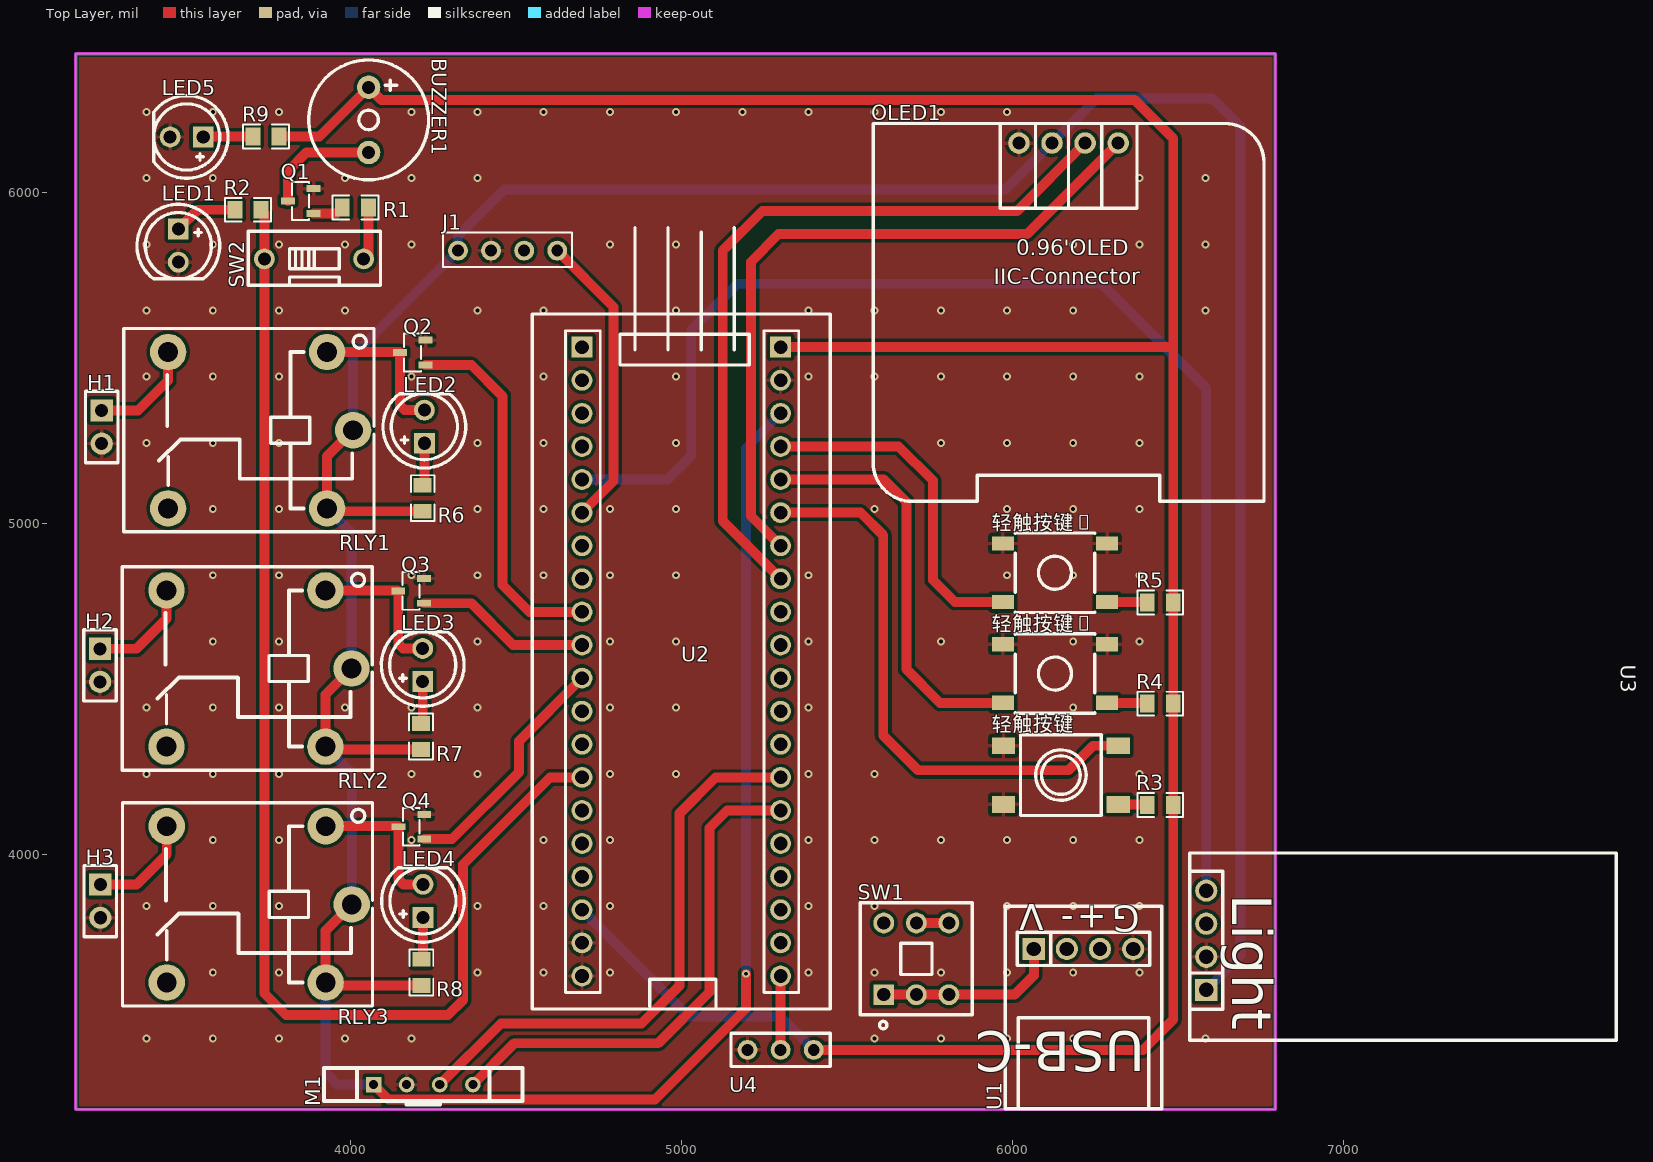
[diagram p0: Top Layer view]
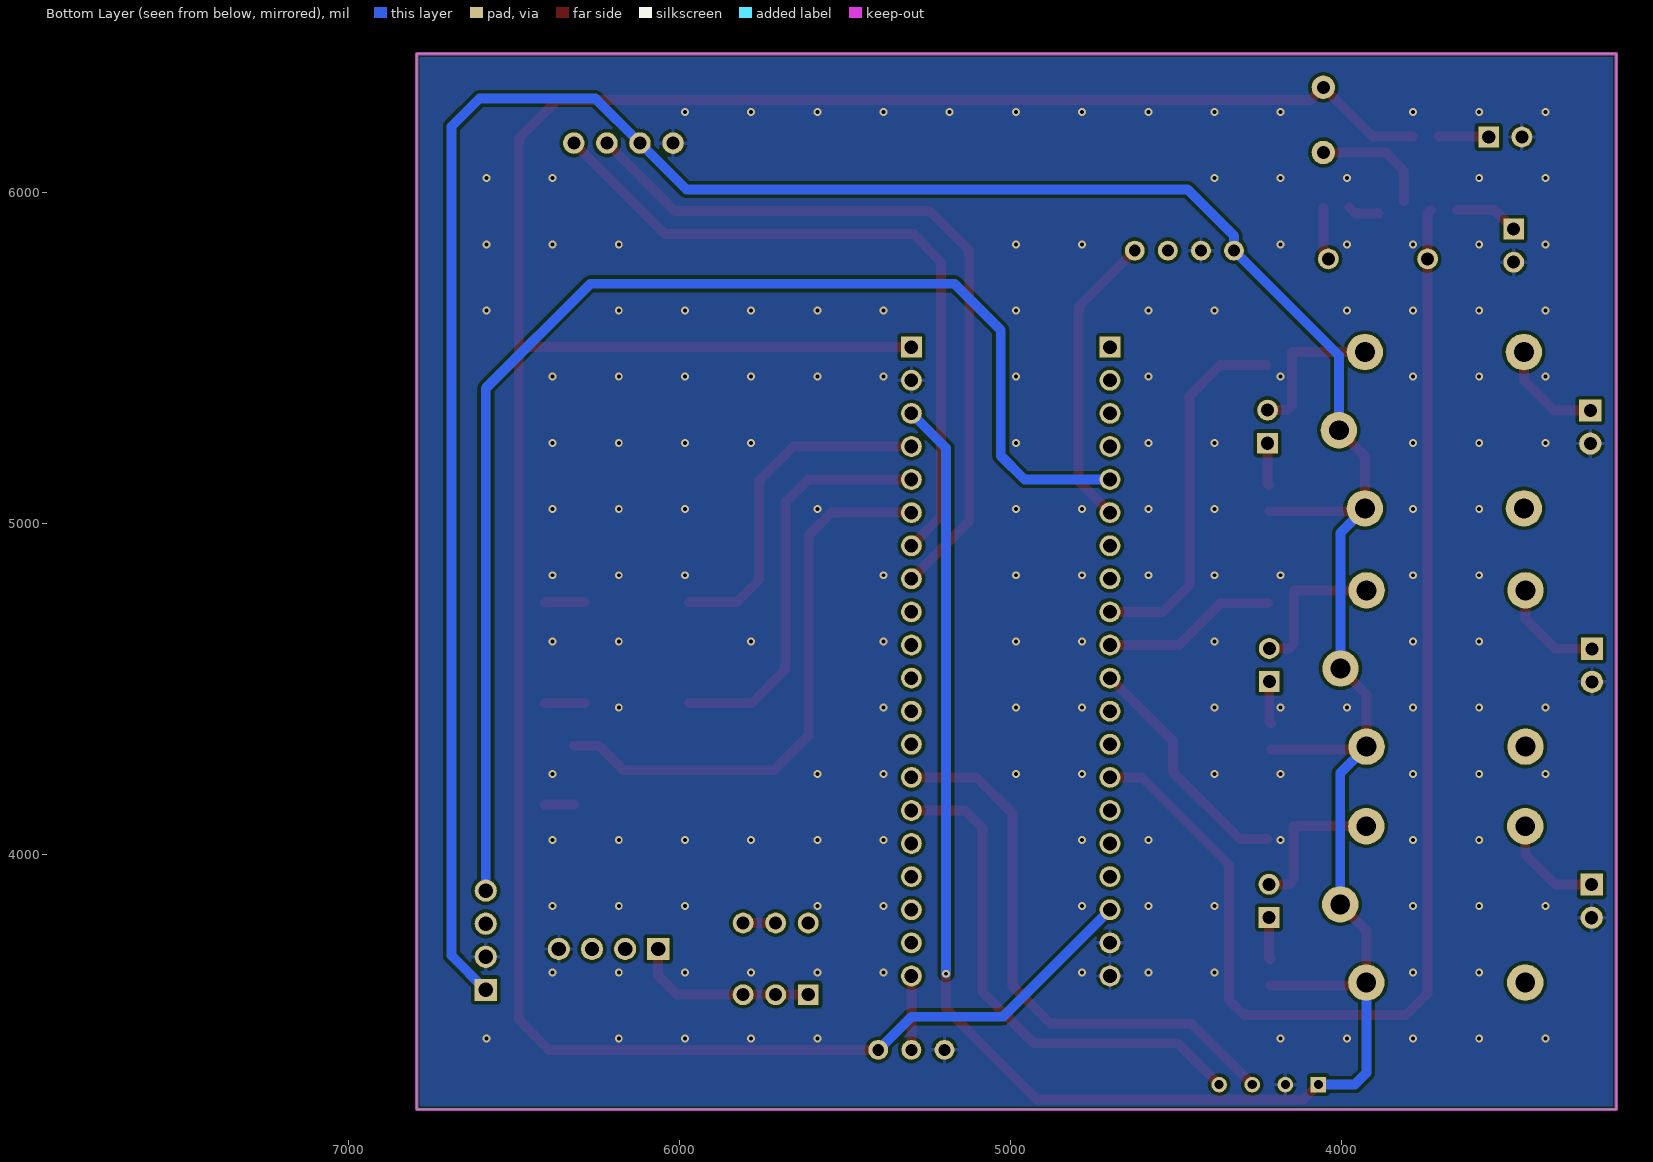
[diagram p1: Bottom Layer view, seen from below]
# Altium PCB MISC51322.pcbdoc
Units mil, origin at the board's own origin, x right, y up, seen from the top; angles counter-clockwise.
Board outline 3625 x 3190 mil, 2 copper layers (Top Layer, Bottom Layer), stack 62.206 mil thick; 37 components, 36 nets, 146 pads, 159 vias.

## Layer stack, top to bottom
Top Solder Mask Layer: solder mask 0.394, Dk 3.3
Top Layer: signal copper 1.379
Dielectric1: surface 59.449, FR4, Dk 4.5
Bottom Layer: signal copper 1.378
Bottom Solder Mask Layer: solder mask 0.394, Dk 3.3

## Board outline
3170,6420 3170,3230 6795,3230 6795,6420

## Design rules (kind name [scope] priority, off if disabled: settings)
BoardOutlineClearance copperThickness2oz_1 [All] p2 off: genericclearance=7.99 ignorepadtopadclearanceinfootprint=FALSE except(0: Arc-SplitContinuation Track-SplitContinuation SMDPad-SplitContinuation THPad-SplitContinuation Via-SplitContinuation Fill-SplitContinuation Region-SplitContinuation Poly-SplitContinuation Text-SplitContinuation Hole-SplitContinuation; 5.98: Arc-CutoutEdge SMDPad-CutoutEdge THPad-CutoutEdge Via-CutoutEdge Fill-CutoutEdge Region-CutoutEdge Text-CutoutEdge; 6.93: Hole-OutlineEdge Hole-CutoutEdge; 10: Poly-OutlineEdge Poly-CutoutEdge; 11.81: Arc-OutlineEdge Track-OutlineEdge SMDPad-OutlineEdge THPad-OutlineEdge Via-OutlineEdge Fill-OutlineEdge Region-OutlineEdge Text-OutlineEdge Track-CutoutEdge)
BoardOutlineClearance copperThickness1oz_1 [All] p4: genericclearance=4.02 ignorepadtopadclearanceinfootprint=FALSE except(0: Arc-SplitContinuation Track-SplitContinuation SMDPad-SplitContinuation THPad-SplitContinuation Via-SplitContinuation Fill-SplitContinuation Region-SplitContinuation Poly-SplitContinuation Text-SplitContinuation Hole-SplitContinuation; 6: SMDPad-CutoutEdge THPad-CutoutEdge Via-CutoutEdge Fill-CutoutEdge Region-CutoutEdge Text-CutoutEdge; 6.93: Hole-OutlineEdge Hole-CutoutEdge; 10: Poly-OutlineEdge Poly-CutoutEdge; 11.8: Arc-OutlineEdge Track-OutlineEdge SMDPad-OutlineEdge THPad-OutlineEdge Via-OutlineEdge Fill-OutlineEdge Region-OutlineEdge Text-OutlineEdge; 11.81: Arc-CutoutEdge Track-CutoutEdge)
Clearance copperThickness2oz [All] p1 off: gap=7.99 ignorepadtopadclearanceinfootprint=FALSE except(5.98: SMDPad-Track SMDPad-SMDPad THPad-Track SMDPad-THPad THPad-THPad Track-Via SMDPad-Via THPad-Via Via-Via Fill-Track Region-Track Fill-SMDPad Region-SMDPad Fill-THPad Region-THPad Fill-Via Region-Via Fill-Fill Fill-Region Region-Region Arc-Track Arc-SMDPad Arc-THPad Arc-Via Fill-Arc Region-Arc Arc-Arc Text-Track SMDPad-Text Text-THPad Text-Via Fill-Text Region-Text Arc-Text Text-Text; 6.93: Hole-Track Hole-SMDPad Hole-THPad Hole-Via Fill-Hole Region-Hole Hole-Arc Hole-Text; 10: Poly-Track Poly-SMDPad Poly-THPad Poly-Via Poly-Fill Poly-Region Poly-Poly Poly-Arc Poly-Text Poly-Hole)
Clearance copperThickness1oz [All] p3: gap=4.02 ignorepadtopadclearanceinfootprint=FALSE except(5.98: SMDPad-Track SMDPad-SMDPad THPad-Track SMDPad-THPad THPad-THPad Track-Via SMDPad-Via THPad-Via Via-Via Fill-Track Region-Track Fill-SMDPad Region-SMDPad Fill-THPad Region-THPad Fill-Via Region-Via Fill-Fill Fill-Region Region-Region; 6: Arc-Track Arc-SMDPad Arc-THPad Arc-Via Fill-Arc Region-Arc Arc-Arc Text-Track SMDPad-Text Text-THPad Text-Via Fill-Text Region-Text Arc-Text Text-Text; 6.93: Hole-Track Hole-SMDPad Hole-THPad Hole-Via Fill-Hole Region-Hole Hole-Arc Hole-Text; 10: Poly-Track Poly-SMDPad Poly-THPad Poly-Via Poly-Fill Poly-Region Poly-Poly Poly-Arc Poly-Text Poly-Hole)
DiffPairsRouting differentialPair [All] p1: maxlimit=6 minlimit=6 mostfreqgap=6 toplayer_minwidth=5 toplayer_prefwidth=10 toplayer_maxwidth=100 toplayer_mingap=6 toplayer_prefgap=6 toplayer_maxgap=6 bottomlayer_minwidth=5 bottomlayer_prefwidth=10 bottomlayer_maxwidth=100 bottomlayer_mingap=6 bottomlayer_prefgap=6 bottomlayer_maxgap=6 maxuncoupledlength=10
HoleToHoleClearance otherClearance [All] p1: gap=11.81 allowstackedmicrovias=TRUE
Length netLength [All] p1: minlimit=0 maxlimit=0
MatchedLengths netLengthTolerance [All] p1: tolerance=1000
PasteMaskExpansion pasteMaskExpansion [All] p1: expansion=0
PlaneConnect innerPlane [All] p1: planeconnectstyle=Relief reliefexpansion=20 reliefentries=4 reliefconductorwidth=10 reliefairgap=10
PolygonConnect copperRegion [(InNet('GND'))] p1: connectstyle=Relief reliefconductorwidth=10 reliefentries=4 polygonreliefangle="90 Angle" airgapwidth=10 via.connectstyle=Relief via.reliefconductorwidth=10 via.reliefentries=4 via.polygonreliefangle="90 Angle" via.airgapwidth=10
RoutingVias viaSize [All] p1: holewidth=12.01 width=24.02 viastyle="Through Hole" minholewidth=11.81 minwidth=19.68 maxholewidth=248.03 maxwidth=393.7
SolderMaskExpansion solderMaskExpansion [IsVia] p1: expansion=-1000 istentingtop=TRUE
SolderMaskExpansion solderMaskExpansion [All] p2: expansion=2 istentingtop=FALSE
Width copperThickness2oz_2 [All] p1 off: maxlimit=100 minlimit=8 preferedwidth=10
Width copperThickness1oz_2 [All] p2: maxlimit=100 minlimit=5 preferedwidth=10

## Components (designator, comment, footprint, x,y, rotation, side; value= is the part's Value field where it differs from the comment)
BUZZER1 "3kHz" BUZ-TH_BD9.0-P5.00-D0.6-FD 4055,6220 r270 top
H1 "" HDR-TH_2P-P2.54-V-F 3248.48,5291.97 r270 top
H2 "" HDR-TH_2P-P2.54-V-F 3243.48,4571.97 r270 top
H3 "" HDR-TH_2P-P2.54-V-F 3244.21,3859.22 r270 top
J1 "土壤湿度传感器模块" Hearder-4 4325,5825 r0 top
LED1 "" LED-TH_5mm 3480,5840 r270 top
LED2 "" LED-TH_5mm 4223.48,5293.03 r90 top
LED3 "" LED-TH_5mm 4218.48,4573.03 r90 top
LED4 "" LED-TH_5mm 4219.21,3860.28 r90 top
LED5 "" LED-TH_5mm 3505.35,6168.51 r180 top
M1 "BT06" BT06 4070,3305 r90 top
OLED1 "" 0.96OLED_4P 6170,6150 r0 top
Q1 "S8050" SOT-23-3_L2.9-W1.3-P1.90-LS2.3-BR 3850,5975 r0 top
Q2 "S8050" SOT-23-3_L2.9-W1.3-P1.90-LS2.3-BR 4188.48,5516.97 r0 top
Q3 "S8050" SOT-23-3_L2.9-W1.3-P1.90-LS2.3-BR 4183.48,4796.97 r0 top
Q4 "S8050" SOT-23-3_L2.9-W1.3-P1.90-LS2.3-BR 4184.21,4084.22 r0 top
R1 "1K" R0805 4015,5955 r180 top
R2 "1K" R0805 3690.35,5948.51 r0 top
R3 "10K" R0805 6446.93,4150.32 r0 top
R4 "10K" R0805 6446.93,4456.02 r0 top
R5 "10K" R0805 6446.93,4761.73 r0 top
R6 "1K" R0805 4218.48,5076.97 r90 top
R7 "1K" R0805 4213.48,4356.97 r90 top
R8 "1K" R0805 4214.21,3644.22 r90 top
R9 "1K" R0805 3745,6170 r0 top
RLY1 "SRD-05VDC-SL-C" RELAY-TH_SRD-XXVDC-XL-C 3728.75,5282.36 r180 top
RLY2 "SRD-05VDC-SL-C" RELAY-TH_SRD-XXVDC-XL-C 3723.75,4562.36 r180 top
RLY3 "SRD-05VDC-SL-C" RELAY-TH_SRD-XXVDC-XL-C 3724.48,3849.61 r180 top
SW1 "自锁开关" SW-TH_6P-L8.5-W8.5-P2.50-LS5.5-BL-2 5710,3685 r0 top
SW2 "拨码" SW-TH_DSWB01LHGET 3890,5800 r90 top
U1 "" USB-type-C模块 6215,3715 r90 top
U2 "CW32F030C8最小系统板" STM32F103C8T6核心板 4999.86,4583.38 r0 top
U3 "" 光敏传感器模块 6535,3735 r270 top
U4 "DS18B20" 3p_2.54 5300,3410 r0 top
轻触按键 "SH-6X6X6.5H-TP" SW-SMD_4P-L6.2-W6.2-P4.50-LS9.5-TL 6146.68,4240.32 r0 top
轻触按键1 "SH-6X6X6.5H-TP" SW-SMD_4P-L6.0-W6.0-P4.50-LS8.8 6128.96,4547.05 r0 top
轻触按键2 "SH-6X6X6.5H-TP" SW-SMD_4P-L6.0-W6.0-P4.50-LS8.8 6128.96,4851.73 r0 top

## Footprints (in the part's own frame and the unit in brackets; to place one, negate y for a bottom-side part, rotate by r counter-clockwise, add the part's x,y. Pads: shape width x height; smd on the part's side, far side on the other; paste and mask are expansions set on the pad)
0.96OLED_4P [mm]
  round 1.65 hole 1 copper offset 0,0: 1(-3.81,-0.001) 2(-1.27,0.002) 3(1.27,0.002) 4(3.81,0.002)
  silkscreen extent -15,-27.5 15,1.5
3p_2.54 [mil]
  round 60 hole 36: 1(-100,0) 2(0,0) 3(100,0)
  silkscreen extent -150,-50 150,50
BT06 [mm]
  rect 1.2x1.2 hole 0.7: 1(0,0)
  round 1.2 hole 0.7: 2(0,-2.54) 3(0,-5.08) 4(0,-7.62)
  silkscreen extent -1.52,-11.43 1.27,3.81
BUZ-TH_BD9.0-P5.00-D0.6-FD [mm]
  round 1.8 hole 1 copper offset 0,0: 1(-2.5,0)
  round 1.8 hole 1: 2(2.5,0)
  silkscreen extent -4.6,-4.6 4.6,4.6
HDR-TH_2P-P2.54-V-F [mm]
  rect 1.7x1.7 hole 1: 1(-1.27,0)
  round 1.7 hole 1: 2(1.27,0)
  silkscreen extent -2.74,-1.25 2.74,1.25
Hearder-4 [mil]
  round 60 hole 36: 1(0,0) 2(100,0) 3(200,0) 4(300,0)
  silkscreen extent -45,-50 345,55
LED-TH_5mm [mm]
  rect 1.6x1.6 hole 1 paste+0 mask+0.051: 1(-1.27,0)
  round 1.6 hole 1 paste+0 mask+0.051: 2(1.27,0)
  silkscreen extent -3.17,-3.17 2.54,3.17
R0805 [mm]
  rect 1.133x1.377 smd paste-100 mask+0.051: 1(-1,0) 2(1,0)
  silkscreen extent -1.76,-0.92 1.76,0.92
RELAY-TH_SRD-XXVDC-XL-C [mil]
  round 110 hole 60: 1(-200.79,-236.22) 2(279.53,-236.2) 3(279.53,236.2) 4(-200.79,236.22) 5(-279.53,0)
  silkscreen extent -342,-307 413,307
SOT-23-3_L2.9-W1.3-P1.90-LS2.3-BR [mm]
  rect 1.07x0.532 smd: 1(0.99,-0.95) 2(0.99,0.95) 3(-0.99,0)
  silkscreen extent -0.66,-1.45 0.64,1.45
STM32F103C8T6核心板 [mil]
  rect 63x63 hole 41.3 paste+4 mask+4: 1(-300,950) 40(300,950)
  round 63 hole 41.3 paste+4 mask+4: 2(-300,850) 3(-300,750) 4(-300,650) 5(-300,550) 6(-300,450) 7(-300,350) 8(-300,250) 9(-300,150) 10(-300,50) 11(-300,-50) 12(-300,-150) 13(-300,-250) 14(-300,-350) 15(-300,-450) 16(-300,-550) 17(-300,-650) 18(-300,-750) 19(-300,-850) 20(-300,-950) 21(300,-950) 22(300,-850) 23(300,-750) 24(300,-650) 25(300,-550) 26(300,-450) 27(300,-350) 28(300,-250) 29(300,-150) 30(300,-50) 31(300,50) 32(300,150) 33(300,250) 34(300,350) 35(300,450) 36(300,550) 37(300,650) 38(300,750) 39(300,850)
  silkscreen extent -450,-1050 450,1312
SW-SMD_4P-L6.0-W6.0-P4.50-LS8.8 [mm]
  rect 1.7x1.1 smd: 1(-4,2.25) 2(-4,-2.25) 3(4,2.25) 4(4,-2.25)
  silkscreen extent -3.05,-3.05 3.05,3.05
SW-SMD_4P-L6.2-W6.2-P4.50-LS9.5-TL [mm]
  rect 1.8x1.3 smd: 1(-4.4,2.25) 2(4.4,2.25) 3(-4.4,-2.25) 4(4.4,-2.25)
  silkscreen extent -3.1,-3.1 3.1,3.1
SW-TH_6P-L8.5-W8.5-P2.50-LS5.5-BL-2 [mm]
  rect 1.6x1.6 hole 1: 1(-2.5,-2.75)
  round 1.6 hole 1: 2(0,-2.75) 3(2.5,-2.75) 4(2.5,2.75) 5(0,2.75) 6(-2.5,2.75)
  silkscreen extent -4.3,-5.36 4.3,4.3
SW-TH_DSWB01LHGET [mm]
  round 1.6 hole 1: 1(0,3.81) 2(0,-3.81)
  silkscreen extent -2.02,-5.11 2.13,5.05
USB-type-C模块 [mm]
  rect 1.7x1.7 hole 1.1: 1(0,3.81)
  round 1.7 hole 1.1: 2(0,1.27) 3(0,-1.27) 4(0,-3.81)
  silkscreen extent -12.27,-6 3.27,6
光敏传感器模块 [mm]
  rect 1.7x1.7 hole 1.1: 1(3.652,1.296)
  round 1.7 hole 1.1: 2(1.112,1.296) 3(-1.428,1.296) 4(-3.968,1.296)
  silkscreen extent -6.86,0.03 7.51,32.77

## Via types
v1: diameter 24.02, hole 12, Top Layer to Bottom Layer, 159 vias

## Nets (pads, with @x,y where several pads share a name; then routed paths per layer and width w, separated by ;. In a path a pad name is that pad's centre, name@x,y a point inside that pad or via, vN(x,y) a via of type N, cw(c..) or ccw(c..) an arc to the next point about the centre after c; other vN are vias at no path point)
$1N6: SW1.4 SW1.5 | length 98.4
  Top Layer w30: SW1.5 SW1.4
$1N8: BUZZER1.2 Q1.3 | length 358
  Top Layer w30: Q1.3 3811.01,6066.02 3866.57,6121.57 BUZZER1.2
$1N10: Q1.1 R1.2 | length 93.9
  Top Layer w30: Q1.1 3958.23,5937.6 R1.2
$1N14: LED1.1 R2.1 | length 195.2
  Top Layer w30: LED1.1 3538.51,5948.51 R2.1
$1N15: R1.1 SW2.2 | length 161
  Top Layer w30: SW2.2 4054.37,5814.37 R1.1
$1N23: R3.1 轻触按键.4 | length 88.2
  Top Layer w30: 轻触按键.4 6406.14,4151.73 R3.1
$1N38: R4.1 轻触按键1.4 | length 122.1
  Top Layer w30: 轻触按键1.4 6405.12,4458.47 R4.1
$1N42: R5.1 轻触按键2.4 | length 121.7
  Top Layer w30: 轻触按键2.4 6406.14,4763.15 R5.1
$1N54: LED2.2 Q2.3 RLY1.1 | length 460.1
  Top Layer w30: RLY1.1 4147.89,5518.58 Q2.3 4149.5,5357.52 4163.99,5343.03 LED2.2
$1N59: LED2.1 R6.2 | length 128.8
  Top Layer w30: R6.2 4223.48,5121.34 LED2.1
$1N61: H1.1 RLY1.2 | length 324.2
  Top Layer w30: H1.1 3358.49,5341.97 3449.22,5432.7 RLY1.2
$1N64: H2.1 RLY2.2 | length 324.2
  Top Layer w30: H2.1 3353.49,4621.97 3444.22,4712.7 RLY2.2
$1N67: LED3.1 R7.2 | length 128.8
  Top Layer w30: R7.2 4218.48,4401.34 LED3.1
$1N70: LED3.2 Q3.3 RLY2.1 | length 460.1
  Top Layer w30: RLY2.1 4142.89,4798.58 Q3.3 4144.5,4637.52 4158.99,4623.03 LED3.2
$1N72: H3.1 RLY3.2 | length 324.2
  Top Layer w30: H3.1 3354.22,3909.22 3444.95,3999.95 RLY3.2
$1N75: LED4.1 R8.2 | length 128.8
  Top Layer w30: R8.2 4219.21,3688.59 LED4.1
$1N78: LED4.2 Q4.3 RLY3.1 | length 460.1
  Top Layer w30: RLY3.1 4143.62,4085.83 Q4.3 4145.23,3924.77 4159.72,3910.28 LED4.2
$1N87: LED5.1 R9.1 | length 150.9
  Top Layer w30: LED5.1 3556.85,6170 R9.1
+3.3V: BUZZER1.1 R3.2 R4.2 R5.2 R9.2 U2.18 U2.40 U4.3 | length 8676
  Top Layer w30: R9.2 3906.57,6170 BUZZER1.1 4093.43,6280 6370,6280 6486.3,6163.7 6486.3,5533.25 ; U2.40 6486.17,5533.38 6486.3,5533.25 ; U4.3 6395,3410 6486.3,3501.3 R3.2 R4.2 R5.2 6486.3,5533.25
  Bottom Layer w30: U2.18 5023.24,3510 5300,3510 U4.3
+5V: J1.1 M1.1 OLED1.2 R6.1 R7.1 R8.1 RLY1.4 RLY1.5 RLY2.4 RLY2.5 RLY3.4 RLY3.5 U2.38 U3.1 | length 12182.6
  Top Layer w30: RLY2.5 3924.54,4483.62 RLY2.4 3933.08,4317.6 R7.1 ; RLY3.5 3925.27,3770.87 RLY3.4 3933.81,3604.85 R8.1 ; RLY1.5 3929.54,5203.62 RLY1.4 3938.08,5037.6 R6.1 ; M1.1 4115,3260 4920,3260 5195,3535 v1(5195,3640)
  Bottom Layer w30: RLY2.4 4004.01,4246.67 RLY3.5 ; RLY3.4 3925.27,3339.73 3960,3305 M1.1 ; RLY1.4 4003.28,4972.4 RLY2.5 ; RLY1.5 4008.28,5508.28 J1.1 4325,5870 4465,6010 5979.95,6010 6120,6150.05 6254.95,6285 6605,6285 6690,6200 6690,3695.2 U3.1 ; v1(5195,3640) 5195,5228.52 U2.38
GND: H1.2 H2.2 H3.2 J1.2 LED1.2 LED5.2 M1.2 OLED1.1 Q1.2 Q2.2 Q3.2 Q4.2 U1.4 U2.19 U2.20 U2.39 U3.2 U4.1 轻触按键1.1 轻触按键1.3 轻触按键2.1 轻触按键2.3 轻触按键.1 轻触按键.3
  other v1: 3384.1,3444.1 3584.1,3444.1 3784.1,3444.1 3984.1,3444.1 4184.1,3444.1 5584.1,3444.1 5784.1,3444.1 5984.1,3444.1 6184.1,3444.1 6584.1,3444.1 3584.1,3644.1 3784.1,3644.1 4384.1,3644.1 4584.1,3644.1 4784.1,3644.1 5384.1,3644.1 5584.1,3644.1 5784.1,3644.1 5984.1,3644.1 6184.1,3644.1 6384.1,3644.1 3384.1,3844.1 3584.1,3844.1 3784.1,3844.1 4384.1,3844.1 4584.1,3844.1 4784.1,3844.1 5384.1,3844.1 5584.1,3844.1 5984.1,3844.1 6184.1,3844.1 6384.1,3844.1 3584.1,4044.1 3784.1,4044.1 4184.1,4044.1 4584.1,4044.1 4784.1,4044.1 5384.1,4044.1 5584.1,4044.1 5784.1,4044.1 5984.1,4044.1 6184.1,4044.1 6384.1,4044.1 3384.1,4244.1 3584.1,4244.1 3784.1,4244.1 4184.1,4244.1 4384.1,4244.1 4784.1,4244.1 4984.1,4244.1 5384.1,4244.1 5584.1,4244.1 6384.1,4244.1 3384.1,4444.1 3584.1,4444.1 3784.1,4444.1 3984.1,4444.1 4184.1,4444.1 4384.1,4444.1 4784.1,4444.1 4984.1,4444.1 5384.1,4444.1 6184.1,4444.1 3584.1,4644.1 3784.1,4644.1 4384.1,4644.1 4784.1,4644.1 4984.1,4644.1 5384.1,4644.1 5784.1,4644.1 6184.1,4644.1 6384.1,4644.1 3584.1,4844.1 3784.1,4844.1 4184.1,4844.1 4384.1,4844.1 4584.1,4844.1 4784.1,4844.1 4984.1,4844.1 5384.1,4844.1 5984.1,4844.1 6184.1,4844.1 6384.1,4844.1 3584.1,5044.1 3784.1,5044.1 4384.1,5044.1 4584.1,5044.1 4784.1,5044.1 4984.1,5044.1 5584.1,5044.1 5984.1,5044.1 6184.1,5044.1 6384.1,5044.1 3384.1,5244.1 3584.1,5244.1 3784.1,5244.1 4384.1,5244.1 4584.1,5244.1 4984.1,5244.1 5784.1,5244.1 5984.1,5244.1 6184.1,5244.1 6384.1,5244.1 3384.1,5444.1 3584.1,5444.1 3784.1,5444.1 4184.1,5444.1 4584.1,5444.1 4984.1,5444.1 5384.1,5444.1 5584.1,5444.1 5784.1,5444.1 5984.1,5444.1 6184.1,5444.1 6384.1,5444.1 3384.1,5644.1 3584.1,5644.1 3784.1,5644.1 3984.1,5644.1 4384.1,5644.1 4584.1,5644.1 4984.1,5644.1 5384.1,5644.1 5584.1,5644.1 5784.1,5644.1 5984.1,5644.1 6184.1,5644.1 6584.1,5644.1 3384.1,5844.1 3584.1,5844.1 3784.1,5844.1 3984.1,5844.1 4184.1,5844.1 4784.1,5844.1 4984.1,5844.1 6184.1,5844.1 6384.1,5844.1 6584.1,5844.1 3384.1,6044.1 3584.1,6044.1 3984.1,6044.1 4184.1,6044.1 4384.1,6044.1 6384.1,6044.1 6584.1,6044.1 3384.1,6244.1 3584.1,6244.1 3784.1,6244.1 4184.1,6244.1 4384.1,6244.1 4584.1,6244.1 4784.1,6244.1 4984.1,6244.1 5184.1,6244.1 5384.1,6244.1 5584.1,6244.1 5784.1,6244.1 5984.1,6244.1
IN_5V: SW1.1 SW1.2 SW1.3 U1.1 | length 557.6
  Top Layer w30: SW1.1 SW1.2 SW1.3 6006.73,3576.73 6065,3635 U1.1
PA0: U2.5 U3.4 | length 4002.5
  Bottom Layer w30: U2.5 4958.38,5133.38 5030,5205 5030,5585 5170,5725 6270,5725 6586.02,5408.98 U3.4
PA1: J1.4 U2.6 | length 901.4
  Top Layer w30: J1.4 4795,5655 4795,5128.52 U2.6
PA4: Q2.1 U2.9 | length 1115.4
  Top Layer w30: Q2.1 4365.43,5479.57 4460,5385 4460,4815 4541.62,4733.38 U2.9
PA5: Q3.1 U2.10 | length 529.7
  Top Layer w30: Q3.1 4365.43,4759.57 4491.62,4633.38 U2.10
PA6: Q4.1 U2.11 | length 733
  Top Layer w30: Q4.1 4306.82,4046.82 4510,4250 4510,4343.52 U2.11
PA9_TXD: M1.4 U2.26 | length 1562.9
  Top Layer w30: M1.4 4495,3430 4930,3430 5085,3585 5085,4080 5138.38,4133.38 U2.26
PA10_RXD: M1.3 U2.27 | length 1719
  Top Layer w30: M1.3 4455,3490 4880,3490 4995,3605 4995,4125 5103.38,4233.38 U2.27
PB1: R2.2 SW2.1 U2.14 | length 3897.3
  Top Layer w30: R2.2 3740,5938.23 SW2.1 3740,3580 3805,3515 4295,3515 4340,3560 4340,3970 4603.38,4233.38 U2.14
PB5: OLED1.3 U2.33 | length 2293.7
  Top Layer w30: U2.33 5125,5008.24 5125,5825 5245,5945 6014.95,5945 OLED1.3@6220,6150.05
PB6: OLED1.4 U2.34 | length 2153.6
  Top Layer w30: U2.34 5210,5023.24 5210,5791.1 5293.9,5875 6044.95,5875 OLED1.4@6320,6150.05
PB7: U2.35 轻触按键.2 | length 1727.5
  Top Layer w30: U2.35 5541.62,5033.38 5610,4965 5610,4360 5715,4255 6170,4255 6243.9,4328.9 轻触按键.2
PB8: U2.36 轻触按键1.2 | length 1247
  Top Layer w30: U2.36 5611.62,5133.38 5680,5065 5680,4560 5781.53,4458.47 轻触按键1.2
PB9: U2.37 轻触按键2.2 | length 1042.1
  Top Layer w30: U2.37 5656.62,5233.38 5760,5130 5760,4830 5826.85,4763.15 轻触按键2.2
PB12: U2.21 U4.2 | length 223.4
  Top Layer w30: U2.21 5299.86,3410.14 U4.2
pads on no net: J1.3 RLY1.3 RLY2.3 RLY3.3 SW1.6 U1.2 U1.3 U2.1 U2.2 U2.3 U2.4 U2.7 U2.8 U2.12 U2.13 U2.15 U2.16 U2.17 U2.22 U2.23 U2.24 U2.25 U2.28 U2.29 U2.30 U2.31 U2.32 U3.3

## Polygon pours and split planes (outlines as drawn)
GND on Top Layer (solid, remove dead copper, pour order 0): 3000,6655 3000,3000 7015,3000 7015,6655
GND on Bottom Layer (solid, remove dead copper, pour order 2): 3095,6580 3095,3105 6935,3105 6935,6580

## Keep-outs
Board Outline Layer:
  the board outline again, w10

## Dimensions
6536.02,4470 to 7830,4470 on Document Layer